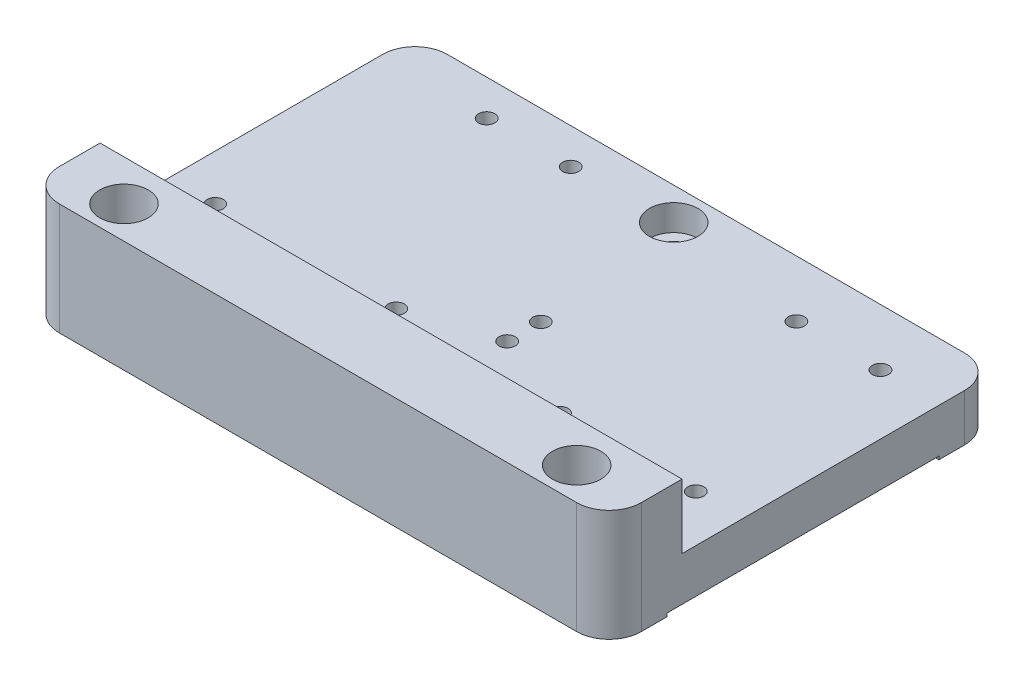
from build123d import *

# Parameters (mm, degrees)
SKETCH1_W             = 90
SKETCH1_H             = 60
BOSS_EXTRUDE1_DEPTH   = 7.3
SKETCH2_W             = 90
SKETCH2_H             = 11.3
BOSS_EXTRUDE2_DEPTH   = 9.98
M3_TAPPED_HOLE1_D     = 2.5
M3_TAPPED_HOLE1_DEPTH = 7.5
M3_TAPPED_HOLE1_TIP   = 0.751075774
FILLET1_R             = 5
SKETCH5_R             = 3.75
CUT_EXTRUDE1_DEPTH    = 14
SKETCH6_R             = 2.1
CUT_EXTRUDE2_DEPTH    = 94.992651145
SKETCH7_W             = 42
SKETCH7_H             = 0.5
CUT_EXTRUDE3_DEPTH    = 108.961191957
M3_TAPPED_HOLE3_D     = 2.5
M3_TAPPED_HOLE3_DEPTH = 8.5
M3_TAPPED_HOLE3_TIP   = 0.751075774


with BuildPart() as part:
    # Sketch1 → Boss-Extrude1 (new body)
    with BuildSketch(Plane(origin=(0, 0, 0), x_dir=(1, 0, 0), z_dir=(0, 1, 0))):
        with Locations((-28.359375, 27.0703125)):
            Rectangle(SKETCH1_W, SKETCH1_H)
    extrude(amount=BOSS_EXTRUDE1_DEPTH)

    # Sketch2 → Boss-Extrude2 (add)
    with BuildSketch(Plane(origin=(0, 7.3, 0), x_dir=(1, 0, 0), z_dir=(0, 1, 0))):
        with Locations((-28.359375, 2.7203125)):
            Rectangle(SKETCH2_W, SKETCH2_H)
    extrude(amount=BOSS_EXTRUDE2_DEPTH)

    # M3 Tapped Hole1
    with Locations(Plane(origin=(0, 7.3, 0), x_dir=(1, 0, 0), z_dir=(0, 1, 0))):
        with Locations((-66.259375, 19.0703125), (-38.259375, 19.0703125), (-56.759375, 51.5503125), (-43.759375, 51.5503125), (-5.619375, 48.3003125), (7.380625, 48.3003125), (-11.619375, 17.7503125), (9.380625, 17.7503125)):
            Hole(M3_TAPPED_HOLE1_D / 2, depth=M3_TAPPED_HOLE1_DEPTH)
            with Locations((0, 0, -(M3_TAPPED_HOLE1_DEPTH + M3_TAPPED_HOLE1_TIP / 2))):  # 118° drill point
                Cone(0, M3_TAPPED_HOLE1_D / 2, M3_TAPPED_HOLE1_TIP, mode=Mode.SUBTRACT)

    # Fillet1
    fillet1_edges = [part.edges().sort_by_distance(p)[0] for p in [
        (-73.359375, 3.65, -57.0703125),
        (16.640625, 3.65, -57.0703125),
        (16.640625, 8.64, 2.9296875),
        (-73.359375, 8.64, 2.9296875),
    ]]
    fillet(fillet1_edges, radius=FILLET1_R)

    # Sketch5 → Cut-Extrude1 (cut)
    with BuildSketch(Plane(origin=(0, 17.28, 0), x_dir=(1, 0, 0), z_dir=(0, 1, 0))):
        with Locations(Location((-28.359375, 52.0703125, 0), (0, 0, 270))):
            Circle(SKETCH5_R)
        with Locations(Location((-63.359375, 2.0703125, 0), (0, 0, 270))):
            Circle(SKETCH5_R)
        with Locations(Location((6.640625, 2.0703125, 0), (0, 0, 90))):
            Circle(SKETCH5_R)
    extrude(amount=-CUT_EXTRUDE1_DEPTH, mode=Mode.SUBTRACT)

    # Sketch6 → Cut-Extrude2 (cut, through all)
    with BuildSketch(Plane(origin=(0, 3.28, 0), x_dir=(1, 0, 0), z_dir=(0, 1, 0))):
        with Locations(Location((-28.359375, 52.0703125, 0), (0, 0, 270))):
            Circle(SKETCH6_R)
        with Locations(Location((-63.359375, 2.0703125, 0), (0, 0, 270))):
            Circle(SKETCH6_R)
        with Locations(Location((6.640625, 2.0703125, 0), (0, 0, 270))):
            Circle(SKETCH6_R)
    extrude(amount=-CUT_EXTRUDE2_DEPTH, mode=Mode.SUBTRACT)

    # Sketch7 → Cut-Extrude3 (cut, through all)
    with BuildSketch(Plane(origin=(16.640625, 0, 0), x_dir=(0, 0, -1), z_dir=(1, 0, 0))):
        with Locations((27.0703125, 0.25)):
            Rectangle(SKETCH7_W, SKETCH7_H)
    extrude(amount=-CUT_EXTRUDE3_DEPTH, mode=Mode.SUBTRACT)

    # M3 Tapped Hole3
    with Locations(Plane(origin=(0, 7.3, 0), x_dir=(1, 0, 0), z_dir=(0, 1, 0))):
        with Locations((-24.569375, 11.7703125), (-24.569375, 16.9703125), (-25.309375, 23.2703125), (-25.309375, 28.4703125)):
            Hole(M3_TAPPED_HOLE3_D / 2, depth=M3_TAPPED_HOLE3_DEPTH)
            with Locations((0, 0, -(M3_TAPPED_HOLE3_DEPTH + M3_TAPPED_HOLE3_TIP / 2))):  # 118° drill point
                Cone(0, M3_TAPPED_HOLE3_D / 2, M3_TAPPED_HOLE3_TIP, mode=Mode.SUBTRACT)


solid = part.part
